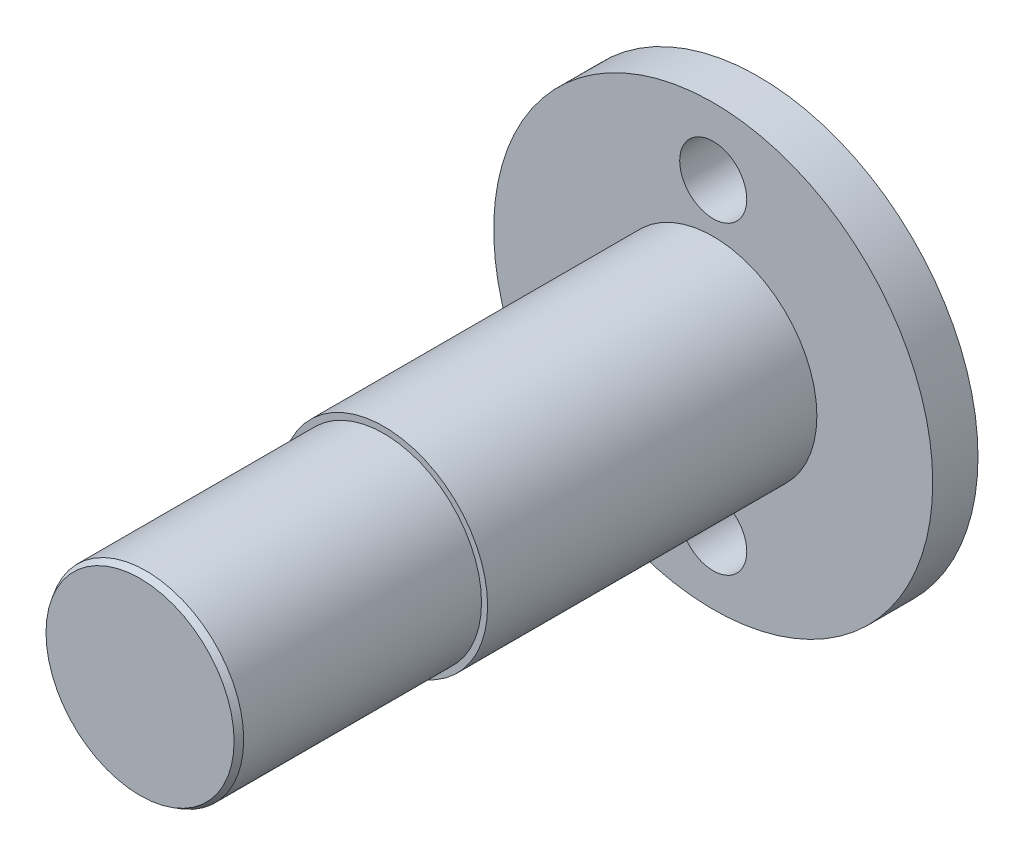
SolidWorks part; units mm, degrees
ref_plane "Front Plane" through (0, 0, 0) normal (0, 0, 1) x (1, 0, 0)
ref_plane "Top Plane" through (0, 0, 0) normal (0, 1, 0) x (1, 0, 0)
ref_plane "Right Plane" through (0, 0, 0) normal (1, 0, 0) x (0, 0, -1)
other "Configuration Table"
sketch "Sketch1" plane through (0, 0, 0) normal (0, 0, 1) x (1, 0, 0)
  circle A0 centre (0, 0) radius 18
  dimension "D1" = 36
extrude "Boss-Extrude1" add sketch "Sketch1" along normal blind 4
sketch "Sketch2" plane through (0, 0, 4) normal (0, 0, 1) x (1, 0, 0)
  circle A0 centre (0, 0) radius 8.5
  dimension "D1" = 17
extrude "Boss-Extrude2" add sketch "Sketch2" along normal blind 27
sketch "Sketch3" plane through (0, 0, 4) normal (0, 0, 1) x (1, 0, 0)
  circle A0 centre (0, 0) radius 8
  dimension "D1" = 16
extrude "Boss-Extrude3" add sketch "Sketch3" along normal blind 20 from surface at 27 starting at face at (8.5, 0, 31)
chamfer "Chamfer1" distance 0.5 angle 30 2 edges at (18, 0, 0) (8, 0, 51)
sketch "Sketch4" plane through (0, 0, 0) normal (0, 0, -1) x (-1, 0, 0)
  circle A0 centre (0, 0) radius 12.5 construction
  circle A1 centre (0, 12.5) radius 2.75
  circle A2 centre (0, -12.5) radius 2.75
  dimension "D1" = 25
  dimension "D2" = 5.5
  dimension "D3" = 5.5
extrude "Cut-Extrude1" cut sketch "Sketch4" against normal blind 20
